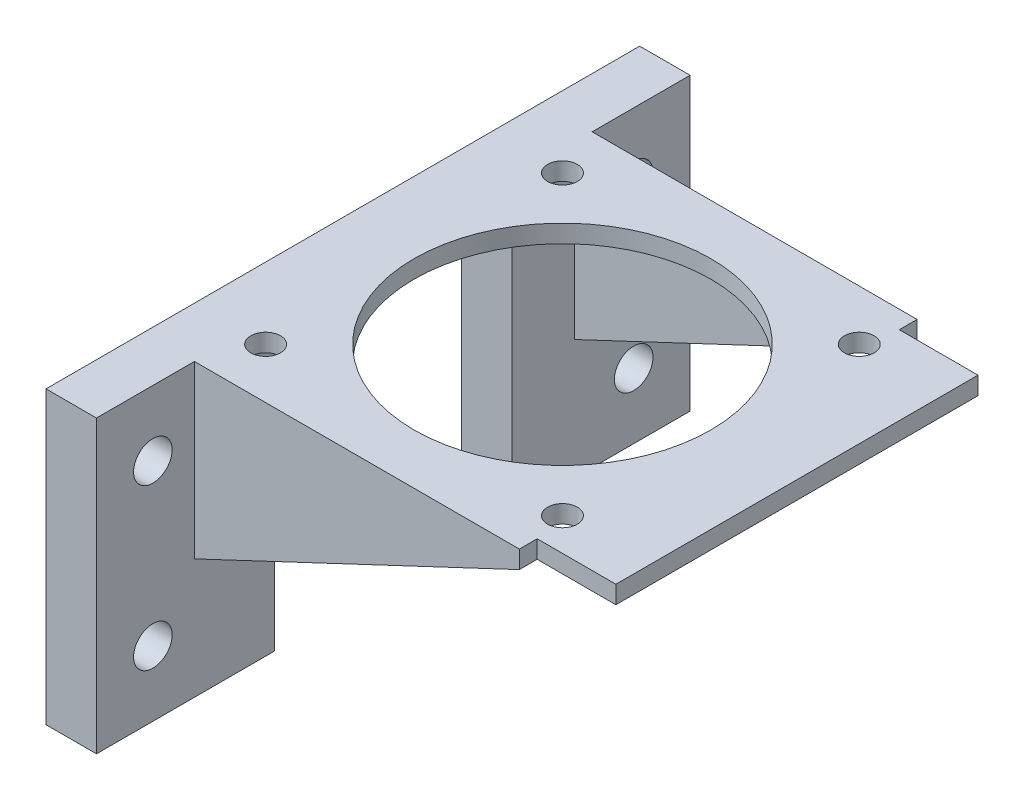
from build123d import *

# Parameters (mm, degrees)
SKETCH_1_W          = 100
SKETCH_1_H          = 49
SKETCH_1_R          = 3.25
EXTRUDE_1_DEPTH     = 8.5
SKETCH_2_W          = 61
SKETCH_2_H          = 3
EXTRUDE_2_DEPTH     = 68
SKETCH_3_R          = 25
CUT_EXTRUDE_1_DEPTH = 68
SKETCH_4_R          = 2.5
CUT_EXTRUDE_2_DEPTH = 68
SKETCH_5_W          = 40
SKETCH_5_H          = 46
CUT_EXTRUDE_3_DEPTH = 15
EXTRUDE_3_DEPTH     = 3


with BuildPart() as part:
    # 草图1 → 凸台-拉伸1 (new body)
    with BuildSketch(Plane(origin=(0, 0, 0), x_dir=(0, 0, -1), z_dir=(1, 0, 0))):
        Rectangle(SKETCH_1_W, SKETCH_1_H)
        with Locations((-40.5, 13.5)):
            Circle(SKETCH_1_R, mode=Mode.SUBTRACT)
        with Locations((40.5, 13.5)):
            Circle(SKETCH_1_R, mode=Mode.SUBTRACT)
        with Locations((40.5, -13.5)):
            Circle(SKETCH_1_R, mode=Mode.SUBTRACT)
        with Locations((-40.5, -13.5)):
            Circle(SKETCH_1_R, mode=Mode.SUBTRACT)
    extrude(amount=EXTRUDE_1_DEPTH)

    # 草图2 → 凸台-拉伸2 (add)
    with BuildSketch(Plane(origin=(8.5, 0, 0), x_dir=(0, 0, -1), z_dir=(1, 0, 0))):
        with Locations((0, 23)):
            Rectangle(SKETCH_2_W, SKETCH_2_H)
    extrude(amount=EXTRUDE_2_DEPTH)

    # 草图3 → 切除-拉伸1 (cut)
    with BuildSketch(Plane.XZ.offset(-21.5)):
        with Locations(Location((37, 0, 0), (0, 0, 270))):
            Circle(SKETCH_3_R)
    extrude(amount=-CUT_EXTRUDE_1_DEPTH, mode=Mode.SUBTRACT)

    # 草图4 → 切除-拉伸2 (cut)
    with BuildSketch(Plane.XZ.offset(-21.5)):
        with Locations(Location((12, 25, 0), (0, 0, 270))):
            Circle(SKETCH_4_R)
        with Locations(Location((62, 25, 0), (0, 0, 270))):
            Circle(SKETCH_4_R)
        with Locations(Location((62, -25, 0), (0, 0, 270))):
            Circle(SKETCH_4_R)
        with Locations(Location((12, -25, 0), (0, 0, 270))):
            Circle(SKETCH_4_R)
    extrude(amount=-CUT_EXTRUDE_2_DEPTH, mode=Mode.SUBTRACT)

    # 草图5 → 切除-拉伸3 (cut)
    with BuildSketch(Plane(origin=(8.5, 0, 0), x_dir=(0, 0, -1), z_dir=(1, 0, 0))):
        with Locations((0, -1.5)):
            Rectangle(SKETCH_5_W, SKETCH_5_H)
    extrude(amount=-CUT_EXTRUDE_3_DEPTH, mode=Mode.SUBTRACT)

    # 草图6 → 凸台-拉伸3 (add)
    with BuildSketch(Plane(origin=(0, 0, -30.5), x_dir=(-1, 0, 0), z_dir=(0, 0, -1))):
        Polygon((-63.240172939, 24.5), (-63.240172939, 21.5), (-8.5, -4.29895258), (-8.5, 24.5), align=None)
    extrude_3 = extrude(amount=EXTRUDE_3_DEPTH)

    # 镜向1: 凸台-拉伸3 across plane
    add(extrude_3.mirror(Plane.XY))


solid = part.part
